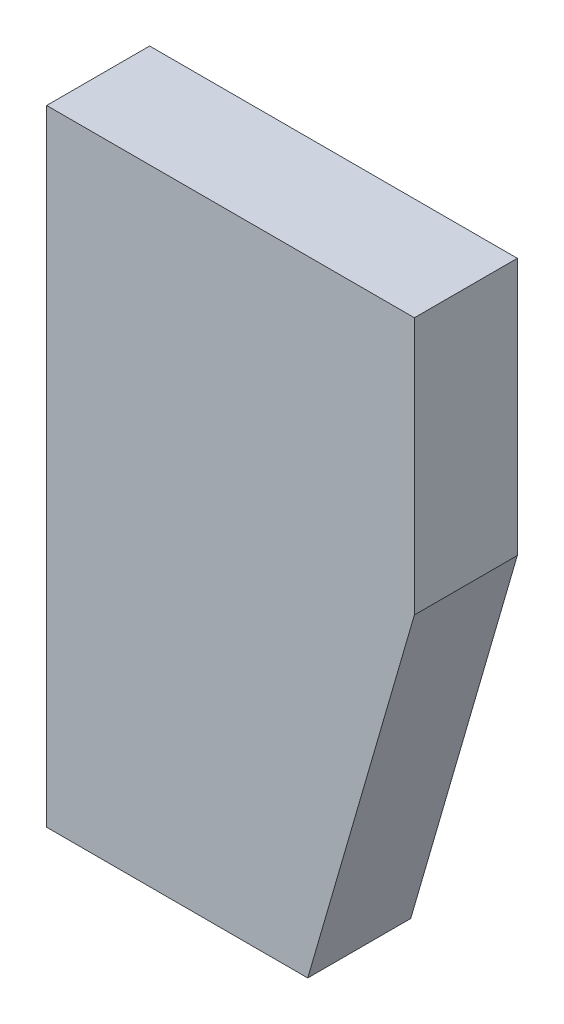
SolidWorks part; units mm, degrees
material "普通碳钢"
ref_plane "前视" through (0, 0, 0) normal (0, 0, 1) x (1, 0, 0)
ref_plane "上视" through (0, 0, 0) normal (0, 1, 0) x (1, 0, 0)
ref_plane "右视" through (0, 0, 0) normal (1, 0, 0) x (0, 0, -1)
sketch "草图1" plane through (0, 0, 0) normal (0, 0, 1) x (1, 0, 0)
  line L0 (-51.7568, 0) -> (56.6216, 0) construction
  line L1 (0, 37.9054) -> (0, -40.2027) construction
  line L2 (0, 0) -> (0, 85)
  line L3 (0, 85) -> (50, 85)
  line L4 (50, 85) -> (50, 50)
  line L5 (50, 50) -> (35.5, 0)
  line L6 (35.5, 0) -> (0, 0)
  dimension "D1" = 35.5
  dimension "D2" = 85
  dimension "D3" = 50
  dimension "15" = 35
extrude "凸台-拉伸1" add sketch "草图1" along normal blind 14
